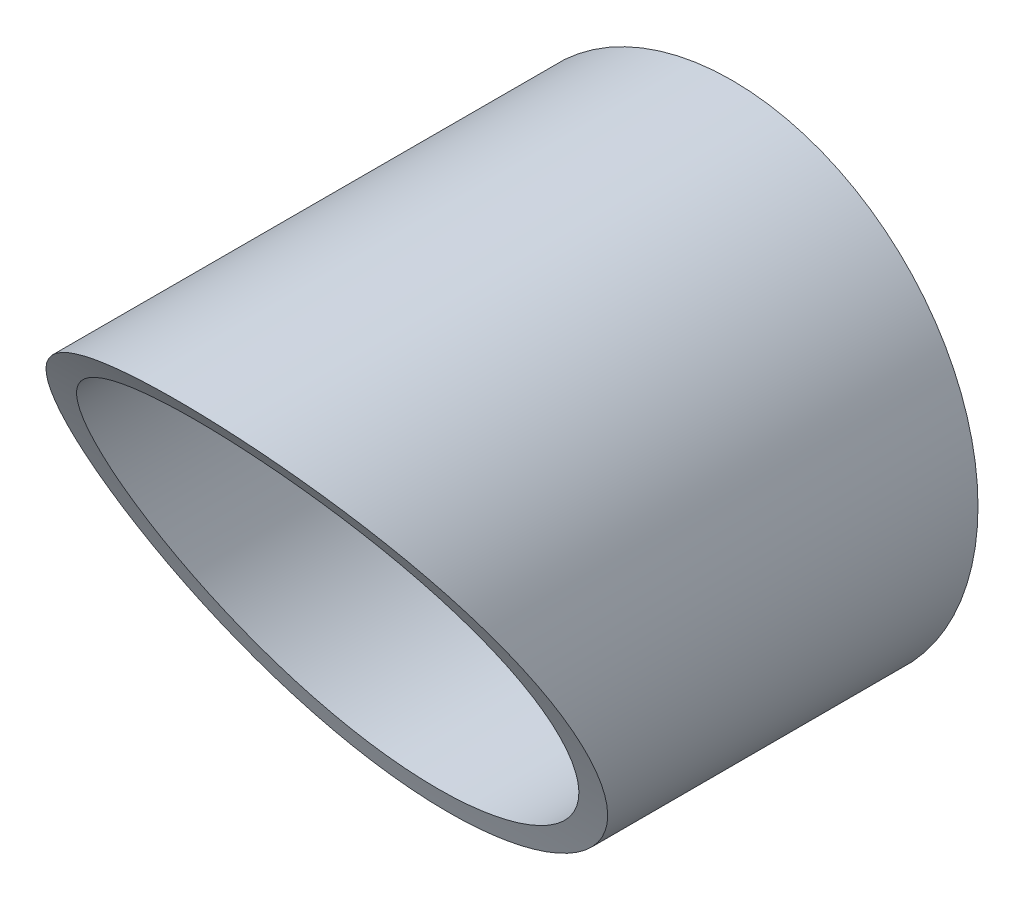
from build123d import *

# Parameters (mm, degrees)
SKETCH1_R           = 38
SKETCH1_R_2         = 34
BOSS_EXTRUDE1_DEPTH = 500
SKETCH2_R           = 379.5
CUT_EXTRUDE1_DEPTH  = 50


with BuildPart() as part:
    # Sketch1 → Boss-Extrude1 (new body)
    with BuildSketch(Plane.XY):
        Circle(SKETCH1_R)
        Circle(SKETCH1_R_2, mode=Mode.SUBTRACT)
    extrude(amount=BOSS_EXTRUDE1_DEPTH)

    # Sketch2 → Cut-Extrude1 (cut, symmetric)
    with BuildSketch(Plane(origin=(0, 0, 0), x_dir=(0, 0, -1), z_dir=(1, 0, 0))):
        with Locations((-395, -181.865334795)):
            Circle(SKETCH2_R)
    extrude(amount=CUT_EXTRUDE1_DEPTH, both=True, mode=Mode.SUBTRACT)


solid = part.part
